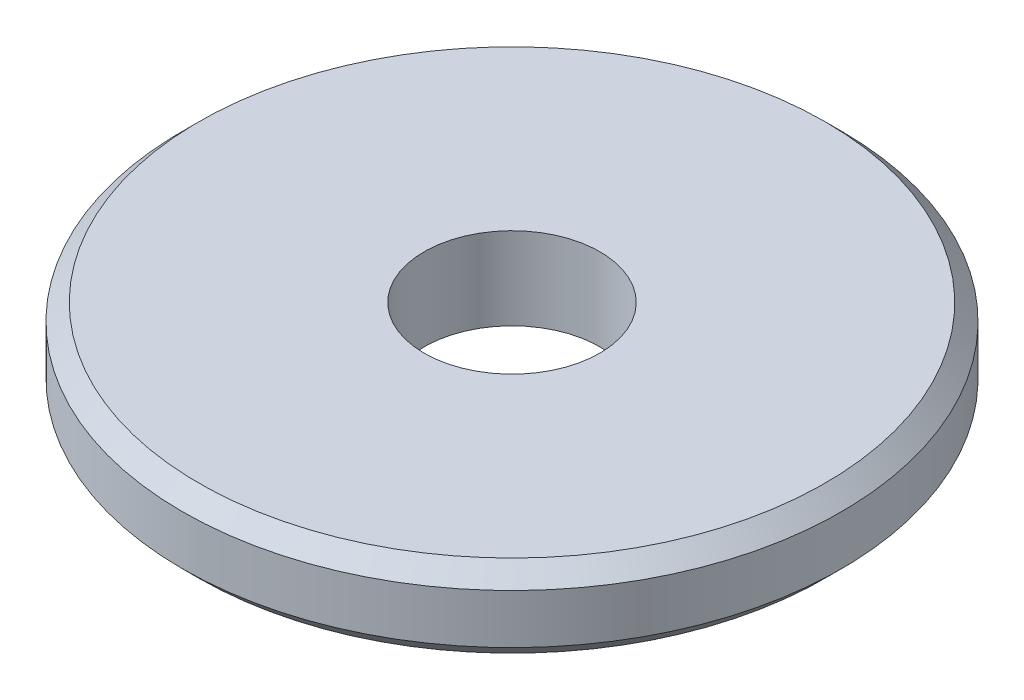
from build123d import *

# Parameters (mm, degrees)
SKETCH1_R           = 6
SKETCH1_R_2         = 1.6
BOSS_EXTRUDE1_DEPTH = 1.5
CHAMFER1_SIZE       = 0.3


with BuildPart() as part:
    # Sketch1 → Boss-Extrude1 (new body)
    with BuildSketch(Plane(origin=(0, 0, 0), x_dir=(1, 0, 0), z_dir=(0, 1, 0))):
        with Locations(Location((0, 0, 0), (0, 0, 270))):
            Circle(SKETCH1_R)
        with Locations(Location((0, 0, 0), (0, 0, 270))):
            Circle(SKETCH1_R_2, mode=Mode.SUBTRACT)
    extrude(amount=BOSS_EXTRUDE1_DEPTH)

    # Chamfer1
    chamfer1_edges = [part.edges().sort_by_distance(p)[0] for p in [
        (0, 0, -6),
        (0, 1.5, -6),
    ]]
    chamfer(chamfer1_edges, length=CHAMFER1_SIZE)


solid = part.part
